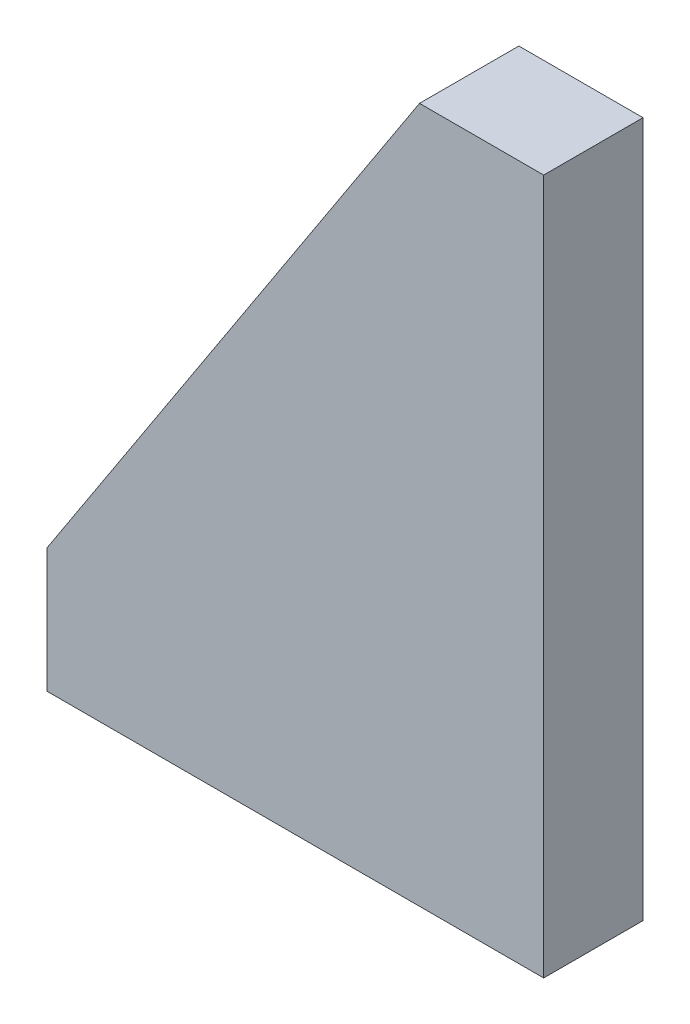
from build123d import *

# Parameters (mm, degrees)
BOSS_EXTRUDE1_DEPTH = 20


with BuildPart() as part:
    # Sketch1 → Boss-Extrude1 (new body)
    with BuildSketch(Plane.XY):
        Polygon((0, 0), (100, 0), (100, 140), (75, 140), (0, 25), align=None)
    extrude(amount=BOSS_EXTRUDE1_DEPTH)


solid = part.part
